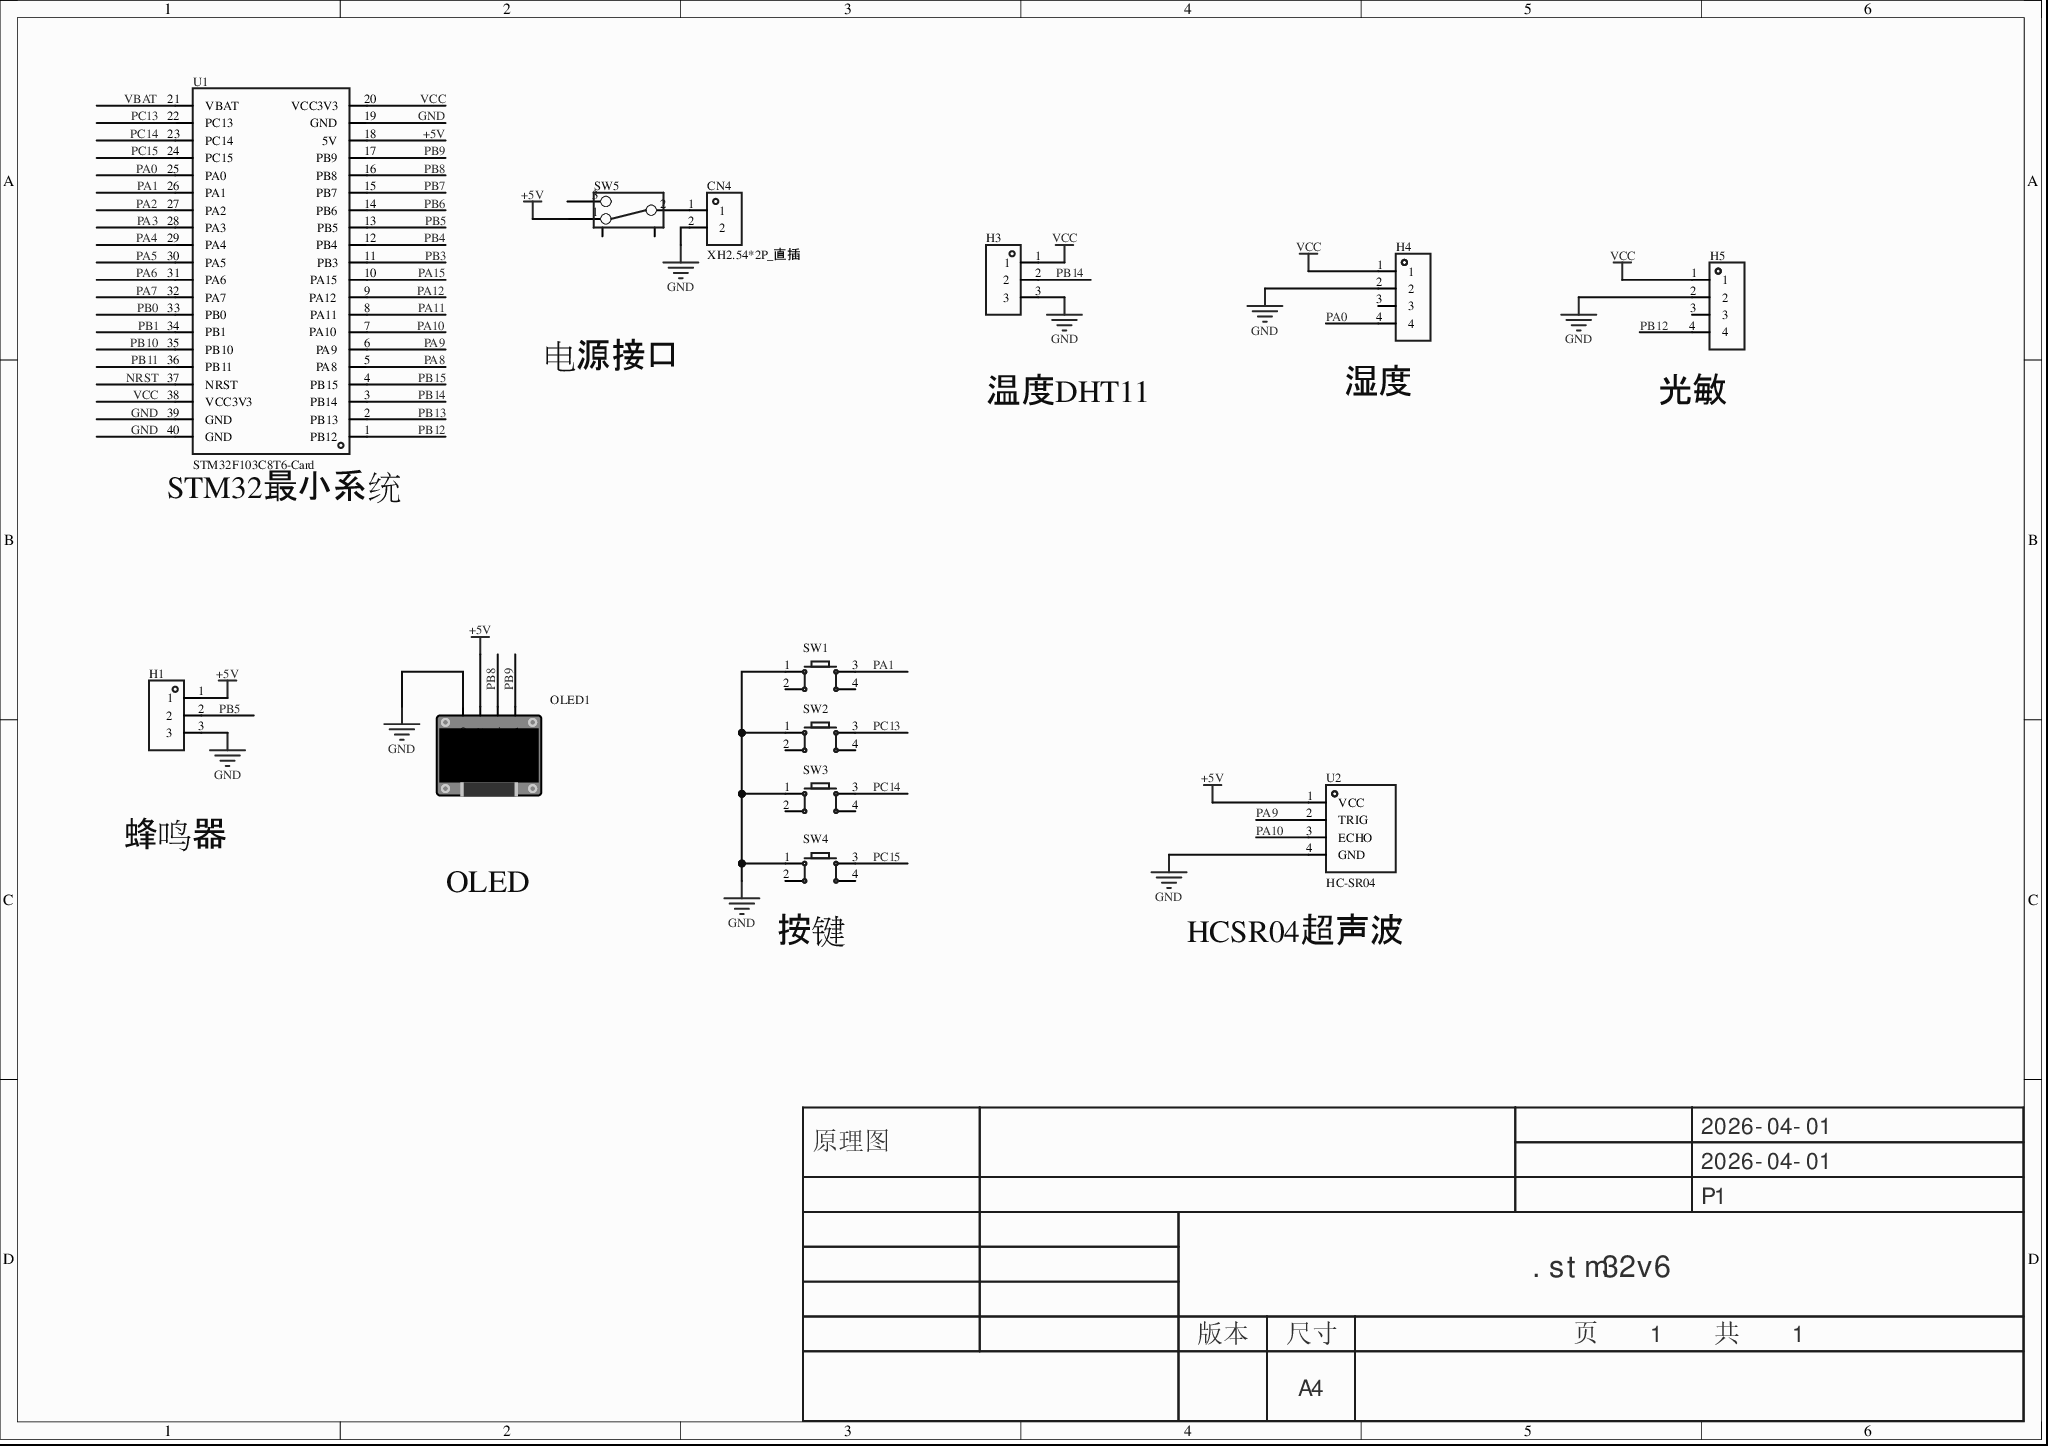
[diagram p0: MISC51673-3.schdoc]
# Altium project MISC51673-2.PrjPcb
1 sheet, 13 parts. Net scope: global (net labels, ports and power ports of the same name join across sheets).
Board file: MISC51673.pcbdoc

## Sheet MISC51673-3.schdoc
size 297 x 209 mm; Version: V1.0; @Project Name: MISC51673; @Page Count: 1; @Update Date: 2026-04-01; @Create Date: 2026-04-01; @Schematic Name: MISC51673; @Page No: 1; @Create Time: 23:22:16; @Update Time: 17:32:40; @Board Name: MISC51673

### Parts
CN4  XH2.54*2P_直插  [CONN-TH_2P-P2.50-XH2.54-2P]
H1  (no value)  [HDR-TH_3P-P2.54-V-F]
H3  (no value)  [HDR-TH_3P-P2.54-V-F]
H4  (no value)  [HDR-TH_4P-P2.54-V-F]
H5  (no value)  [HDR-TH_4P-P2.54-V-F]
OLED1  (no value)  [0.96OLED_4P]
SW1  (no value)  [SW-TH_4P-L6.0-W6.0-P4.50-LS6.5]
SW2  (no value)  [SW-TH_4P-L6.0-W6.0-P4.50-LS6.5]
SW3  (no value)  [SW-TH_4P-L6.0-W6.0-P4.50-LS6.5]
SW4  (no value)  [SW-TH_4P-L6.0-W6.0-P4.50-LS6.5]
SW5  (no value)  [拨动开关]
U1  STM32F103C8T6-Card  [CONN-TH_L53.3-W22.9_STM32F103C8T6-CARD]
U2  HC-SR04  [TH_HC-SR04V]

### Nets
+5V: H1.1 OLED1.2(VCC) SW5.1 U1.18(5V) U2.1(VCC)
GND: CN4.2 H1.3 H3.3 H4.2 H5.2 OLED1.1(GND) SW1.1 SW2.1 SW3.1 SW4.1 U1.19(GND) U1.39(GND) U1.40(GND) U2.4(GND)
VCC: H3.1 H4.1 H5.1 U1.20(VCC3V3) U1.38(VCC3V3)
NRST: U1.37(NRST)
PA0: H4.4 U1.25(PA0)
PA1: SW1.3 U1.26(PA1)
PA2: U1.27(PA2)
PA3: U1.28(PA3)
PA4: U1.29(PA4)
PA5: U1.30(PA5)
PA6: U1.31(PA6)
PA7: U1.32(PA7)
PA8: U1.5(PA8)
PA9: U1.6(PA9) U2.2(TRIG)
PA10: U1.7(PA10) U2.3(ECHO)
PA11: U1.8(PA11)
PA12: U1.9(PA12)
PA15: U1.10(PA15)
PB0: U1.33(PB0)
PB1: U1.34(PB1)
PB3: U1.11(PB3)
PB4: U1.12(PB4)
PB5: H1.2 U1.13(PB5)
PB6: U1.14(PB6)
PB7: U1.15(PB7)
PB8: OLED1.3(SCL) U1.16(PB8)
PB9: OLED1.4(SDA) U1.17(PB9)
PB10: U1.35(PB10)
PB11: U1.36(PB11)
PB12: H5.4 U1.1(PB12)
PB13: U1.2(PB13)
PB14: H3.2 U1.3(PB14)
PB15: U1.4(PB15)
PC13: SW2.3 U1.22(PC13)
PC14: SW3.3 U1.23(PC14)
PC15: SW4.3 U1.24(PC15)
VBAT: U1.21(VBAT)
NetCN4_1: CN4.1 SW5.2

Not connected (* = marked no-connect by the designer): H4 3; H5 3; SW1 2 4; SW2 2 4; SW3 2 4; SW4 2 4; SW5 3 4 5

### Notes on the sheet
- 电源接口
- 温度DHT11
- (near H4) 湿度
- (near H5) 光敏
- (near U1) STM32最小系统
- 蜂鸣器
- OLED
- (near SW4) 按键
- (near U2) HCSR04超声波
- Labels drawn without touching a wire or pin: VCC
- 2026-04-01
- 原理图
- P1
- .stm32v6
- 版本
- 尺寸
- A4
- 页    1    共    1

### Library data of the parts
CN4 = XH2.54*2P_直插: 3D Model: 325c595e30db4df8abe76612dd40b0fa0819f05c4eef4c71ace90d822a990e87; 3D Model Transform: 295.275,228.346,0,180,0,0,-0.002,-20.079,-137.795; AddInBom: yes; Symbol: XH2.54*2P_直插; Device: XH2.54*2P_直插; LCSC Part Name: XH2.54*2P_直插; Supplier Part: C9900008615; Manufacturer Part: XH2.54*2P_直插; Supplier Footprint: XH2.54_2P; JLCPCB Part Class: Extended Part; Supplier: LCSC; ConvertToPcb: yes; FootprintName: CONN-TH_2P-P2.50-XH2.54-2P; ModelName: CONN-TH_2P-P2.50-XH2.54-2P
H1 H3 = HDR-F_2.54_1x3P: Symbol: PM254V-11-03-H85; 3D Model: f3b3cc5aae9641bf9e56fc160cef875b; 3D Model Transform: 299.9994,100,0,0,0,0,0,0,-118.11; ConvertToPcb: yes; ModelName: HDR2.54-F-LI-1X3P; Device: HDR-F_2.54_1x3P; Supplier Part: C541850; Supplier Footprint: 插件; AddInBom: yes; FootprintName: HDR-TH_3P-P2.54-V-F
H4 = HDR-F_2.54_1x4P: Symbol: 2.54-1*4P母; ConvertToPcb: yes; ModelId: d187812051054f85879fcaa51a310d8e0819f05c4eef4c71ace90d822a990e87; ModelTransform: 419.6842,98.464,0,0,0,0,0,0,-118.11; Device: HDR-F_2.54_1x4P; AddInBom: yes; SupplierPart: C2718488; Supplier Footprint: 插件; FootprintName: HDR-TH_4P-P2.54-V-F; ModelName: HDR-TH_4P-P2.54-V-F
H5 = HDR-F_2.54_1x4P: Symbol: 2.54-1*4P母; 3D Model: d187812051054f85879fcaa51a310d8e0819f05c4eef4c71ace90d822a990e87; 3D Model Transform: 419.6842,98.464,0,0,0,0,0,0,-118.11; ConvertToPcb: yes; Device: HDR-F_2.54_1x4P; Supplier Part: C2718488; Supplier Footprint: 插件; AddInBom: yes; FootprintName: HDR-TH_4P-P2.54-V-F; ModelName: HDR-TH_4P-P2.54-V-F
OLED1 = 0.96OLED模块_4P: ConvertToPcb: yes; ModelId: 79c000fdb68d45a296c2e9bedf4f9055; ModelTransform: 1393.69792,1318.895,0,0,0,0,0,-560.079,-137.795; Symbol: 0.96OLED模块_4P; Device: 0.96OLED模块_4P; AddInBom: yes; FootprintName: 0.96OLED_4P; Supplier Footprint: 插件; ModelName: 0.96OLED_4P
SW1-SW4 = Key_TH_6x6x6: 触点电流:50mA;额定电压(DC):12V;绝缘电阻:100MΩ;电路结构:单刀单掷;安装方式:直插;按钮形状:圆形按钮;按钮/盖帽颜色:黑色;作用力:260gf@±30gf;工作温度:-25℃~+70℃;引脚样式:PC引脚;开关长度:6mm;开关宽度:6mm;开关高度:6mm;带支架:否;; Symbol: 轻触按键; AddInBom: yes; ModelId: 20eee248bc684ccd8cbdbb1d0d91ec6f0819f05c4eef4c71ace90d822a990e87; ModelName: SW-TH_4P-L6.0-W6.0-H5.0-LS6.5-P4.50; ModelTransform: 236.22,323.03,0,90,0,0,0,0,-137.795; Device: Key_TH_6x6x6; ConvertToPcb: yes; FootprintName: SW-TH_4P-L6.0-W6.0-P4.50-LS6.5; Supplier Footprint: 插件
SW5 = 拨动开关_正: ConvertToPcb: yes; ModelId: 4321fe59a4074cbfb4989553f297c68f0819f05c4eef4c71ace90d822a990e87; ModelName: SW-TH_SS-12D02-VG4; ModelTransform: 370.09,208.7,472.35,0,0,0,0,0,-110; Symbol: 拨动开关; Device: 拨动开关_正; AddInBom: yes; Supplier Footprint: 插件; FootprintName: 拨动开关
U1 = STM32F103C8T6-Card: AddInBom: yes; Symbol: STM32F103C8T6-CARD; Device: STM32F103C8T6-Card; LCSC Part Name: STM32F103C8T6-Card; SupplierPart: C9900077949; ManufacturerPart: STM32F103C8T6-Card; Supplier Footprint: 插件; Supplier: LCSC; ConvertToPcb: yes; FootprintName: CONN-TH_L53.3-W22.9_STM32F103C8T6-CARD
U2 = HC-SR04: Manufacturer: Universal Microelectronics; AddInBom: yes; Symbol: HC-SR04; Device: HC-SR04; LCSC Part Name: HC-SR04; SupplierPart: C19857336; ManufacturerPart: HC-SR04; Supplier Footprint: -; JLCPCB Part Class: 扩展库; Datasheet: https://atta.szlcsc.com/upload/public/pdf/source/20240122/47B8E374E428935B7962A2189EF91AAC.pdf; Supplier: LCSC; ConvertToPcb: yes; FootprintName: TH_HC-SR04V